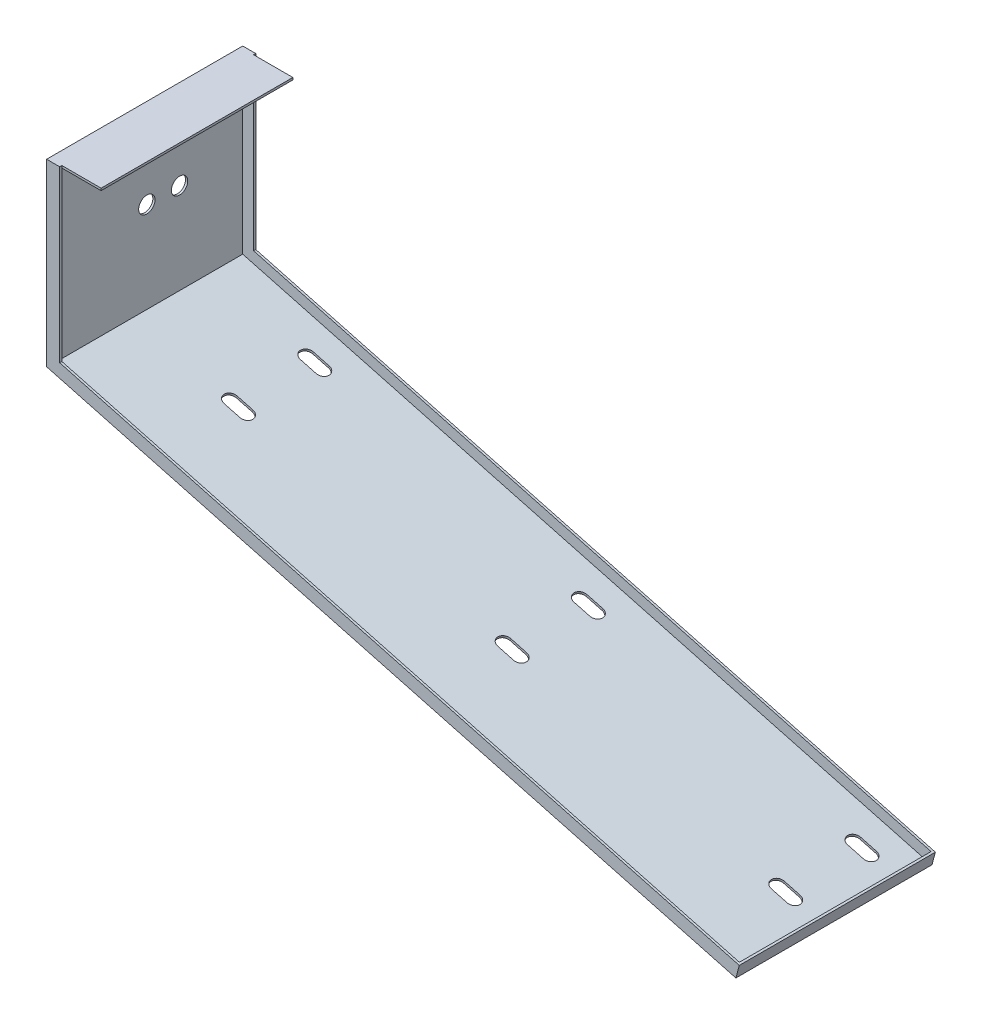
SolidWorks part; units mm, degrees
material "Plain Carbon Steel"
ref_plane "Front Plane" through (0, 0, 0) normal (0, 0, 1) x (1, 0, 0)
ref_plane "Top Plane" through (0, 0, 0) normal (0, 1, 0) x (1, 0, 0)
ref_plane "Right Plane" through (0, 0, 0) normal (1, 0, 0) x (0, 0, -1)
sketch "Sketch1" plane through (0, 0, 0) normal (0, 0, 1) x (1, 0, 0)
  line L0 (0, 0) -> (0, 165)
  line L1 (0, 0) -> (632.6814, -169.5265)
  line L2 (0, 165) -> (48, 165)
  dimension "D1" = 165
  dimension "D2" = 655
  dimension "D3" = 105
  dimension "D4" = 48
extrude "Extrude-Thin1" add sketch "Sketch1" along normal blind 176 thin
sketch "Sketch2" plane through (0, 0, 176) normal (0, 0, 1) x (1, 0, 0)
  line L0 (0, 165) -> (0, 0)
  line L1 (0, 0) -> (632.6814, -169.5265)
  line L2 (632.6814, -169.5265) -> (0, 0) construction
extrude "Extrude-Thin2" add sketch "Sketch2" along normal blind 2 thin thin type one direction reverse wall 12
sketch "Sketch3" plane through (0, 0, 0) normal (0, 0, -1) x (-1, 0, 0)
  line L0 (0, 165) -> (0, 0)
  line L1 (0, 0) -> (-632.6814, -169.5265)
extrude "Extrude-Thin3" add sketch "Sketch3" along normal blind 2 thin
sketch "Sketch4" plane through (0.5176, 1.9319, 0) normal (0.2588, 0.9659, 0) x (0.9659, -0.2588, 0)
  line L1 (655, 0) -> (1.5347, 0) construction
  line L2 (655, -176) -> (653, -176)
  line L3 (655, -176) -> (655, 0)
  line L4 (655, 0) -> (653, 0)
  line L5 (653, -176) -> (653, 0)
  dimension "D1" = 2
extrude "Boss-Extrude1" add sketch "Sketch4" along normal blind 10
sketch "Sketch5" plane through (0, 0, 0) normal (-0.2588, -0.9659, 0) x (0.9659, -0.2588, 0)
  line L0 (611.5, 28) -> (626.5, 28) construction
  line L1 (611.5, 34) -> (626.5, 34)
  line L2 (611.5, 22) -> (626.5, 22)
  line L3 (0, -2) -> (655, -2) construction
  line L4 (655, 178) -> (655, -2) construction
  arc A0 (611.5, 34) -> (611.5, 22) centre (611.5, 28) ccw
  arc A1 (626.5, 22) -> (626.5, 34) centre (626.5, 28) ccw
  point P2 (619, 28)
  dimension "D4" = 6
  dimension "D1" = 30
  dimension "D2" = 36
  dimension "D3" = 15
extrude "Cut-Extrude1" cut sketch "Sketch5" against normal blind 2
pattern_linear "LPattern1" count 3 spacing 260 along (-0.9659, 0.2588, 0) count 2 spacing 70 along (0, 0, 1) of "Cut-Extrude1"
sketch "Sketch6" plane through (2, 0, 0) normal (1, 0, 0) x (0, 0, -1)
  line L0 (-28, 139.0347) -> (-28, 124.0347) construction
  line L1 (-22, 139.0347) -> (-22, 124.0347)
  line L2 (-34, 139.0347) -> (-34, 124.0347)
  line L3 (-176, 1.5347) -> (0, 1.5347) construction
  line L4 (2, 165) -> (2, 9.2079) construction
  arc A0 (-22, 139.0347) -> (-34, 139.0347) centre (-28, 139.0347) ccw
  arc A1 (-34, 124.0347) -> (-22, 124.0347) centre (-28, 124.0347) ccw
  point P2 (-28, 131.5347)
  dimension "D4" = 6
  dimension "D1" = 130
  dimension "D2" = 30
  dimension "D3" = 15
extrude "Cut-Extrude2" cut sketch "Sketch6" against normal blind 2
pattern_linear "LPattern2" count 2 spacing 70 along (0, 0, 1) of "Cut-Extrude2"
sketch "Sketch7" plane through (0, 0, 0) normal (-1, 0, 0) x (0, 0, 1)
  line L0 (-2, 165) -> (-2, 0) construction
  line L1 (178, 0) -> (-2, 0) construction
  circle A0 centre (88, 85) radius 7.5
  dimension "D3" = 15
  dimension "D1" = 90
  dimension "D2" = 85
extrude "Cut-Extrude3" cut sketch "Sketch7" against normal blind 2
pattern_linear "LPattern3" count 2 spacing 30 along (0, 0, -1) of "Cut-Extrude3"
